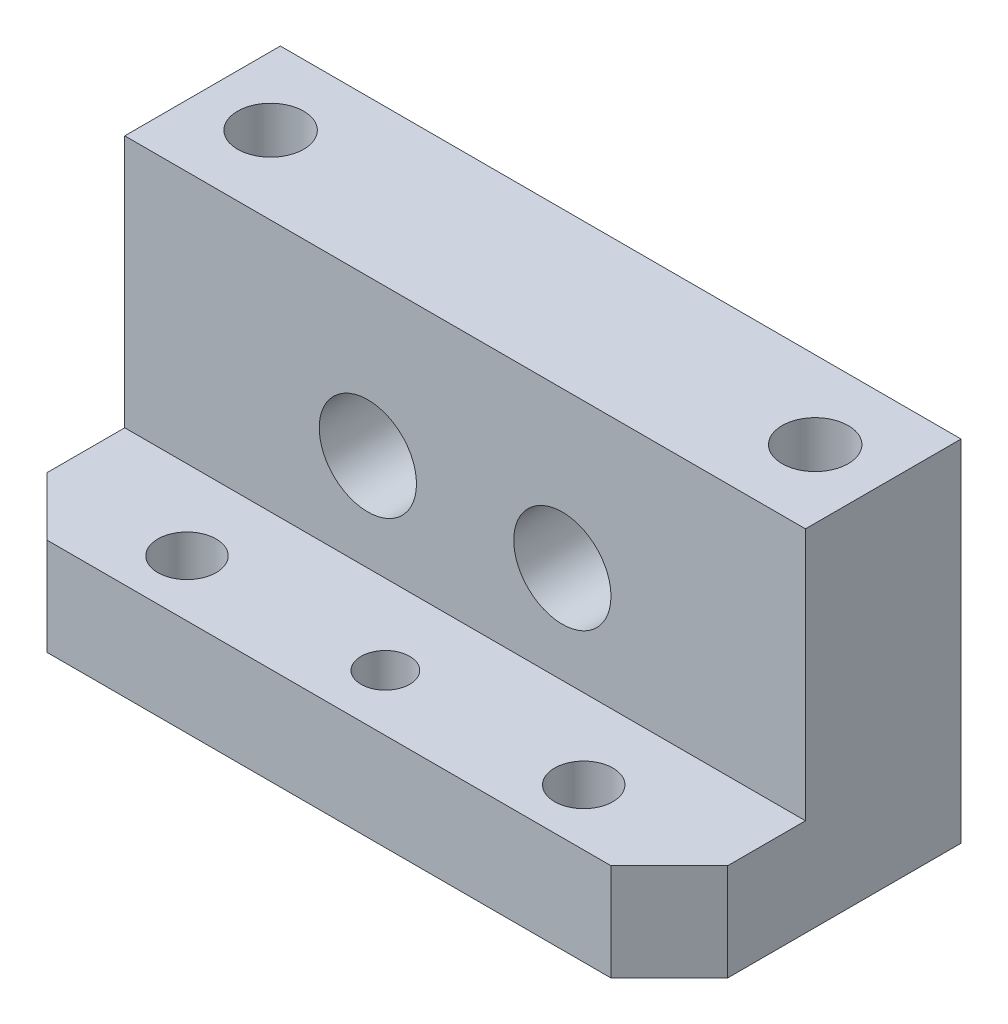
SolidWorks part; units mm, degrees
ref_plane "Front Plane" through (0, 0, 0) normal (0, 0, 1) x (1, 0, 0)
ref_plane "Top Plane" through (0, 0, 0) normal (0, 1, 0) x (1, 0, 0)
ref_plane "Right Plane" through (0, 0, 0) normal (1, 0, 0) x (0, 0, -1)
sketch "Sketch1" plane through (0, 0, 0) normal (0, 0, 1) x (1, 0, 0)
  line L1 (-17.5, 9) -> (17.5, 9)
  line L2 (-17.5, 9) -> (-17.5, -9)
  line L3 (-17.5, -9) -> (17.5, -9)
  line L4 (17.5, 9) -> (17.5, -9)
  line L5 (-17.5, 9) -> (17.5, -9) construction
  line L6 (-17.5, -9) -> (17.5, 9) construction
  point P0 (0, 0)
  dimension "D1" = 35
  dimension "D2" = 18
extrude "Boss-Extrude1" add sketch "Sketch1" along normal mid plane 15
sketch "Sketch2" plane through (17.5, 0, 0) normal (1, 0, 0) x (0, 0, -1)
  line L0 (7.5, -9) -> (7.5, 9) construction
  line L1 (-7.5, 9) -> (-0.5, 9)
  line L2 (-7.5, 9) -> (-7.5, -4)
  line L3 (-7.5, -4) -> (-0.5, -4)
  line L4 (-0.5, 9) -> (-0.5, -4)
  line L5 (-7.5, -9) -> (7.5, -9) construction
  dimension "D1" = 8
  dimension "D2" = 5
extrude "Cut-Extrude1" cut sketch "Sketch2" against normal through all
hole_wizard "Ø5.0 (5) Diameter Hole1" positions "Sketch4" profile "Sketch3" hole size "Ø5.0" standard "Gb" end condition through all
sketch "Sketch4" plane through (0, 0, 0.5) normal (0, 0, 1) x (1, 0, 0)
  line L0 (0, 0) -> (0, 8.2623) construction
  line L2 (-17.5, 9) -> (17.5, 9) construction
  point P0 (-5, 1)
  point P2 (5, 1)
  dimension "D1" = 10
  dimension "D2" = 8
sketch "Sketch3" plane through (-5, 1, 0.5) normal (1, 0, 0) x (0, -1, 0)
  line L0 (0, 0) -> (0, 8)
  line L1 (0, 8) -> (2.5, 8)
  line L2 (2.5, 8) -> (2.5, 0)
  line L5 (2.5, 0) -> (0, 0)
  line L11 (0, -6.35) -> (0, 107.95) construction
  dimension "通孔孔直径" = 5
  dimension "通孔孔深度" = 8
hole_wizard "Ø3.0 (3) Diameter Hole2" positions "Sketch6" profile "Sketch5" hole size "Ø3.0" standard "Gb"
sketch "Sketch6" plane through (0, -4, 0) normal (0, 1, 0) x (1, 0, 0)
  line L0 (0, 0) -> (0, -5.7238) construction
  line L2 (17.5, 7.5) -> (-17.5, 7.5) construction
  point P0 (10.2, -4.6)
  point P3 (-10.2, -4.6)
  dimension "D1" = 20.4
  dimension "D2" = 12.1
sketch "Sketch5" plane through (10.2, -4, 4.6) normal (1, 0, 0) x (0, 0, 1)
  line L0 (0, 0) -> (0, 3.9013)
  line L1 (0, 3.9013) -> (1.5, 3)
  line L2 (1.5, 3) -> (1.5, 0)
  line L5 (1.5, 0) -> (0, 0)
  line L10 (0, 3.9013) -> (-1.5, 3) construction
  line L11 (0, -6.35) -> (0, 107.95) construction
  dimension "孔直径" = 3
  dimension "孔深度" = 3
  dimension "导头角度" = 118
hole_wizard "M3 Tapped Hole1" positions "Sketch8" profile "Sketch7" tap size "M3" standard "Gb" end condition through all
sketch "Sketch8" plane through (0, -9, 0) normal (0, -1, 0) x (-1, 0, 0)
  line L0 (17.5, 7.5) -> (-17.5, 7.5) construction
  point P0 (0, -4.6)
  dimension "D1" = 12.1
sketch "Sketch7" plane through (0, -9, 4.6) normal (1, 0, 0) x (0, 0, -1)
  line L0 (0, 0) -> (0, 18)
  line L1 (0, 18) -> (1.25, 18)
  line L2 (1.25, 18) -> (1.25, 0)
  line L5 (1.25, 0) -> (0, 0)
  line L11 (0, -6.35) -> (0, 107.95) construction
  dimension "通孔螺纹孔钻头直径" = 2.5
  dimension "通孔螺纹孔钻头深度" = 18
cosmetic thread "Hole Thread1" parameters "D2"=3
hole_wizard "Hole size per socket head cap screw type1" positions "Sketch10" profile "Sketch9" counterbore size "M3" standard "Gb" end condition through all
sketch "Sketch10" plane through (0, -9, 0) normal (0, -1, 0) x (-1, 0, 0)
  line L0 (0, 0) -> (0, 10.3395) construction
  line L2 (17.5, 7.5) -> (-17.5, 7.5) construction
  point P0 (14, 3.5)
  point P2 (-14, 3.5)
  dimension "D1" = 4
  dimension "D2" = 28
sketch "Sketch9" plane through (-14, -9, -3.5) normal (1, 0, 0) x (0, 0, -1)
  line L0 (0, 0) -> (0, 18)
  line L1 (0, 18) -> (1.7, 18)
  line L3 (1.7, 18) -> (1.7, 5)
  line L4 (1.7, 5) -> (3, 5)
  line L5 (3, 5) -> (3, 0)
  line L7 (3, 0) -> (0, 0)
  line L11 (0, -6.35) -> (0, 107.95) construction
  dimension "通孔孔直径" = 3.4
  dimension "通孔孔深度" = 18
  dimension "柱形沉头孔直径" = 6
  dimension "柱形沉头孔深度" = 5
chamfer "Chamfer1" distance 3 angle 45 2 edges at (-17.5, -6.5, 7.5) (17.5, -6.5, 7.5)
